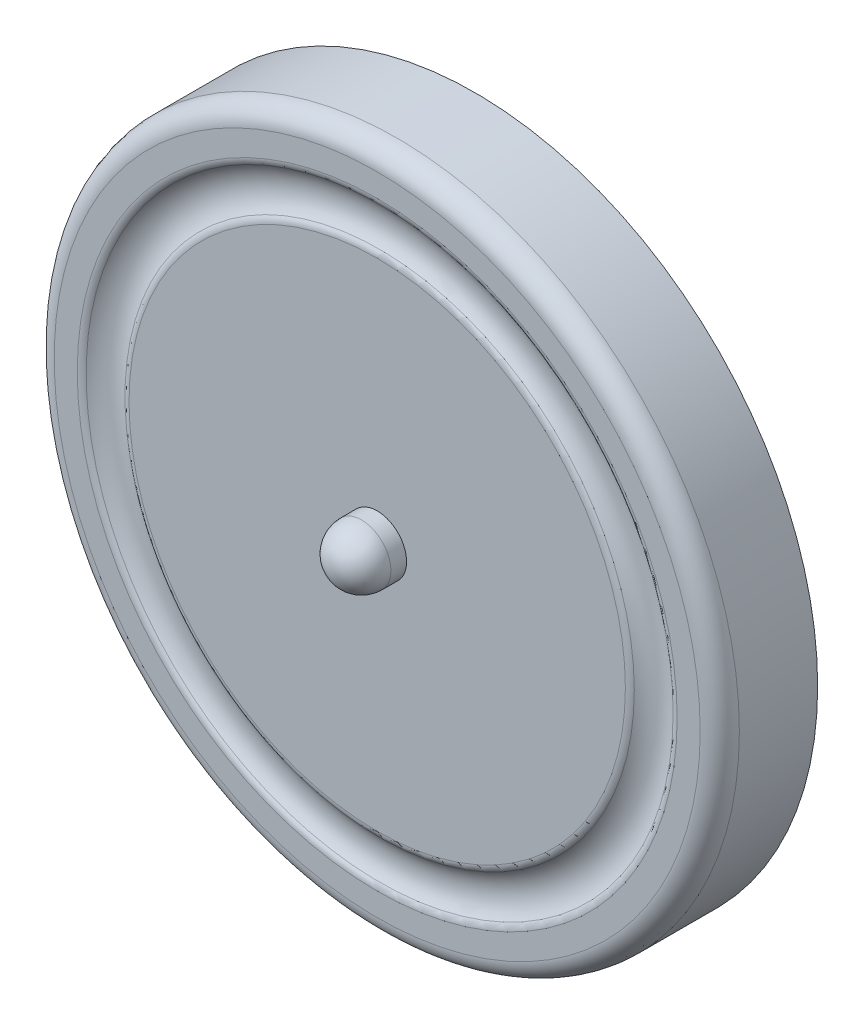
from build123d import *

# Parameters (mm, degrees)
SKETCH1_R           = 17.5
BOSS_EXTRUDE1_DEPTH = 5
SKETCH5_R           = 1.5
FILLET1_R           = 1
FILLET2_R           = 0.5


with BuildPart() as part:
    # Sketch1 → Boss-Extrude1 (new body)
    with BuildSketch(Plane.XY):
        with Locations((-121.531169153, 115.619026916)):
            Circle(SKETCH1_R)
    extrude(amount=BOSS_EXTRUDE1_DEPTH)

    # Sketch2 → Cut-Revolve1 (revolve, cut)
    with BuildSketch(Plane(origin=(-144.568448824, 61.197146719, 0), x_dir=(-0.38982136890031954, -0.9208904931362258, 0), z_dir=(0.9208904931362258, -0.38982136890031954, 0)), mode=Mode.PRIVATE) as cut_revolve1_sk:
        with BuildLine():
            Line((-59.097015989, 0), (-53.597015989, 0))
            Line((-53.597015989, 0), (-53.597015989, -1))
            ThreePointArc((-53.597015989, -1), (-53.889909208, -1.707106781), (-54.597015989, -2))
            Line((-54.597015989, -2), (-59.097015989, -2))
            Line((-59.097015989, -2), (-59.097015989, 0))
        make_face()
    revolve(cut_revolve1_sk.sketch.rotate(Axis((-121.531169153, 115.619026916, 5.87680908), (0, 0, -1)), 337.056615089), axis=Axis((-121.531169153, 115.619026916, 5.87680908), (0, 0, -1)), mode=Mode.SUBTRACT)

    # Sketch5 → Cut-Revolve2 (revolve, cut)
    with BuildSketch(Plane.ZX.offset(115.619026916), mode=Mode.PRIVATE) as cut_revolve2_sk:
        with Locations((6, -107.531169153)):
            Circle(SKETCH5_R)
    revolve(cut_revolve2_sk.sketch.rotate(Axis((-121.531169153, 115.619026916, 5), (0, 0, -1)), 292.943384911), axis=Axis((-121.531169153, 115.619026916, 5), (0, 0, -1)), mode=Mode.SUBTRACT)

    # Fillet1
    fillet1_edges = [part.edges().sort_by_distance(p)[0] for p in [
        (-139.031169153, 115.619026916, 5),
    ]]
    fillet(fillet1_edges, radius=FILLET1_R)

    # Fillet2
    fillet2_edges = [part.edges().sort_by_distance(p)[0] for p in [
        (-126.552834778, 103.756146884, 5),
        (-127.424501858, 101.696973141, 5),
    ]]
    fillet(fillet2_edges, radius=FILLET2_R)

    # Sketch6 → Revolve2 (revolve)
    with BuildSketch(Plane.ZX.offset(115.619026916)):
        with BuildLine():
            Line((5.8, -120.031169153), (4, -120.031169153))
            Line((4, -120.031169153), (4, -121.531169153))
            Line((4, -121.531169153), (7.3, -121.531169153))
            ThreePointArc((7.3, -121.531169153), (6.860660172, -120.470508981), (5.8, -120.031169153))
        make_face()
    revolve(axis=Axis((-121.531169153, 115.619026916, 0), (0, 0, 1)))


with BuildPart() as body_2:
    # Sketch4 → Revolve1 (revolve)
    with BuildSketch(Plane(origin=(-144.568448824, 61.197146719, 0), x_dir=(-0.38982136890031954, -0.9208904931362258, 0), z_dir=(0.9208904931362258, -0.38982136890031954, 0))):
        with BuildLine():
            Line((-59.097015989, -2), (-59.097015989, 3))
            ThreePointArc((-59.097015989, 3), (-56.597015989, 0.5), (-59.097015989, -2))
        make_face()
    revolve(axis=Axis((-121.531169153, 115.619026916, 5), (0, 0, -1)))


solid = Compound([part.part, body_2.part])
